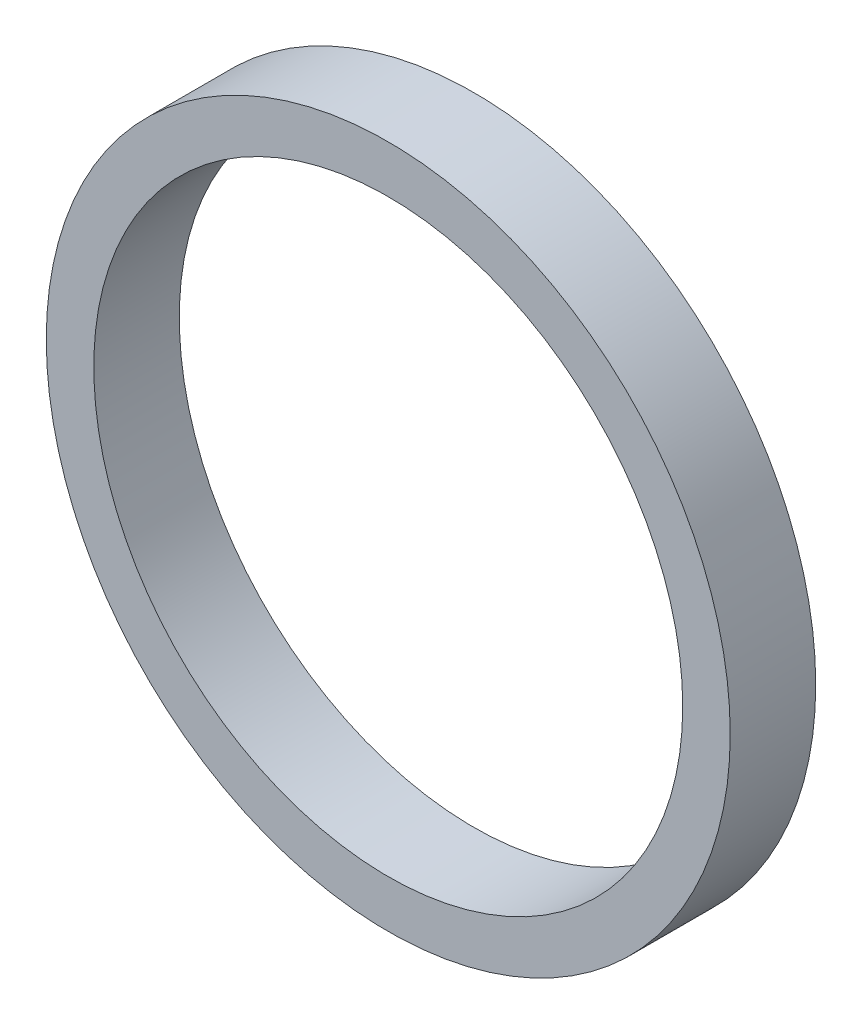
SolidWorks part; units mm, degrees
ref_plane "前视基准面" through (0, 0, 0) normal (0, 0, 1) x (1, 0, 0)
ref_plane "上视基准面" through (0, 0, 0) normal (0, 1, 0) x (1, 0, 0)
ref_plane "右视基准面" through (0, 0, 0) normal (1, 0, 0) x (0, 0, -1)
sketch "草图1" plane through (0, 0, 0) normal (0, 0, 1) x (1, 0, 0)
  circle A0 centre (0, 0) radius 18
  circle A1 centre (0, 0) radius 15.5
extrude "凸台-拉伸1" add sketch "草图1" along normal blind 4.5
